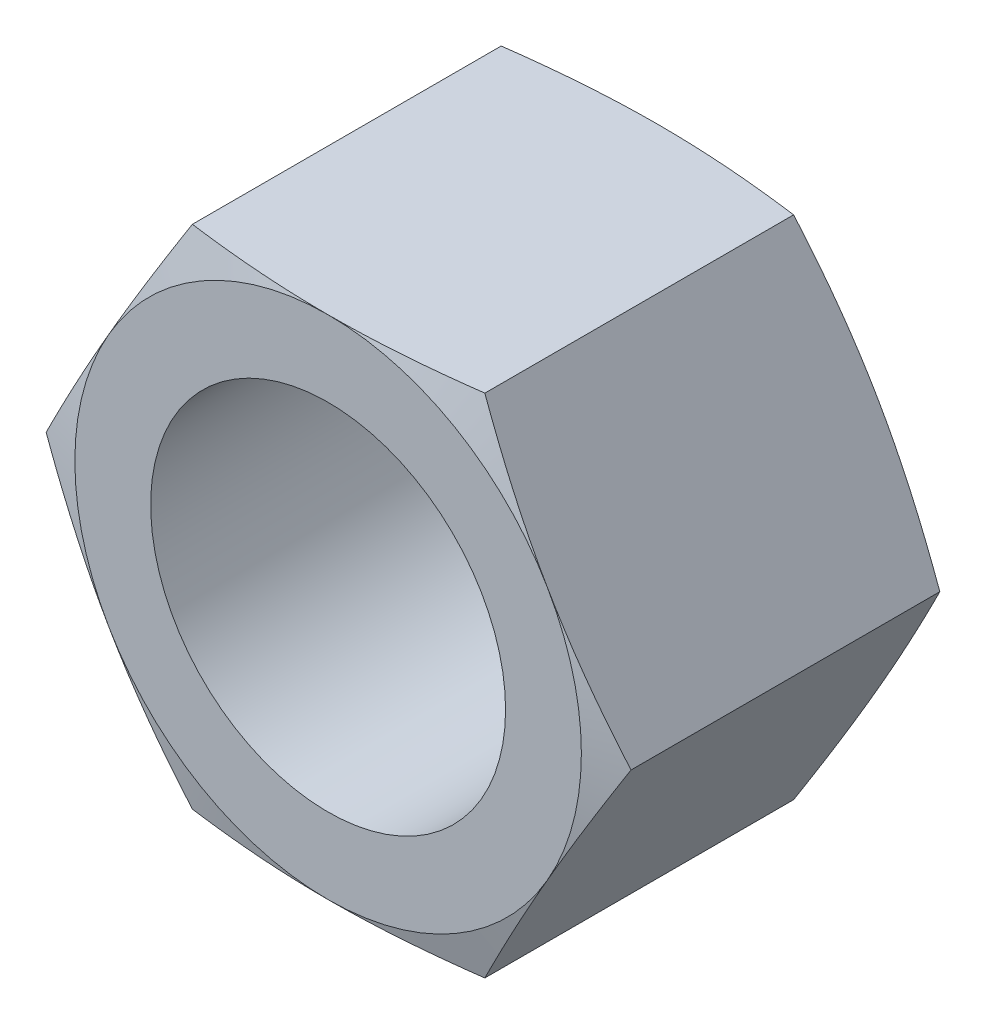
SolidWorks part; units mm, degrees
ref_plane "Plane1" through (0, 0, 0) normal (0, 0, 1) x (1, 0, 0)
ref_plane "Plane2" through (0, 0, 0) normal (0, 1, 0) x (1, 0, 0)
ref_plane "Plane3" through (0, 0, 0) normal (1, 0, 0) x (0, 0, -1)
sketch "dimension sketch" plane through (0, 0, 0) normal (0, 0, 1) x (1, 0, 0)
  line L0 (0, 0) -> (24.1005, 0)
  point P3 (24, 0)
  point P4 (1.5, 0)
  point P5 (39.55, 0)
  point P6 (22.3, 0)
  point P7 (6.4, 0)
  point P8 (36, 0)
sketch "Sketch1" plane through (0, 0, 0) normal (0, 0, 1) x (1, 0, 0)
  line L0 (-26.8088, 0) -> (37.1748, 0) construction
  line L1 (0, 25.0215) -> (0, -25.0215) construction
  line L3 (9.8875, 17.1257) -> (-9.8875, 17.1257)
  line L4 (-9.8875, 17.1257) -> (-19.775, 0)
  line L5 (-19.775, 0) -> (-9.8875, -17.1257)
  line L6 (-9.8875, -17.1257) -> (9.8875, -17.1257)
  line L7 (9.8875, -17.1257) -> (19.775, 0)
  line L8 (19.775, 0) -> (9.8875, 17.1257)
  circle A0 centre (0, 0) radius 17.1257 construction
  circle A1 centre (0, 0) radius 12
extrude "Base-Extrude" add sketch "Sketch1" along normal blind 22.3
cosmetic thread "Cosmetic Thread1" parameters "D2"=25.2
sketch "Sketch2" plane through (0, 0, 0) normal (0, 0, -1) x (-1, 0, 0)
  line L0 (-9.8875, 17.1257) -> (9.8875, 17.1257) construction
  circle A0 centre (0, 0) radius 17.1257
  circle A1 centre (0, 0) radius 12 construction
extrude "Cut-Extrude1" cut sketch "Sketch2" against normal blind 38 draft 75 flip side to cut
sketch "Sketch3" plane through (0, 0, 22.3) normal (0, 0, 1) x (1, 0, 0)
  line L0 (19.775, 0) -> (9.8875, 17.1257) construction
  circle A0 centre (0, 0) radius 17.1257
extrude "Cut-Extrude2" cut sketch "Sketch3" against normal blind 38 draft 75 flip side to cut
chamfer "Chamfer1" [suppressed] distance 0.2 angle 45
equation "\"e@Sketch1\" = \"e@dimension sketch\""
equation "\"D@Sketch1\" = \"D@dimension sketch\""
equation "\"m@Base-Extrude\" = \"m@dimension sketch\""
equation "\"D2@Cosmetic Thread1\" = 1.05 * \"D@dimension sketch\""
